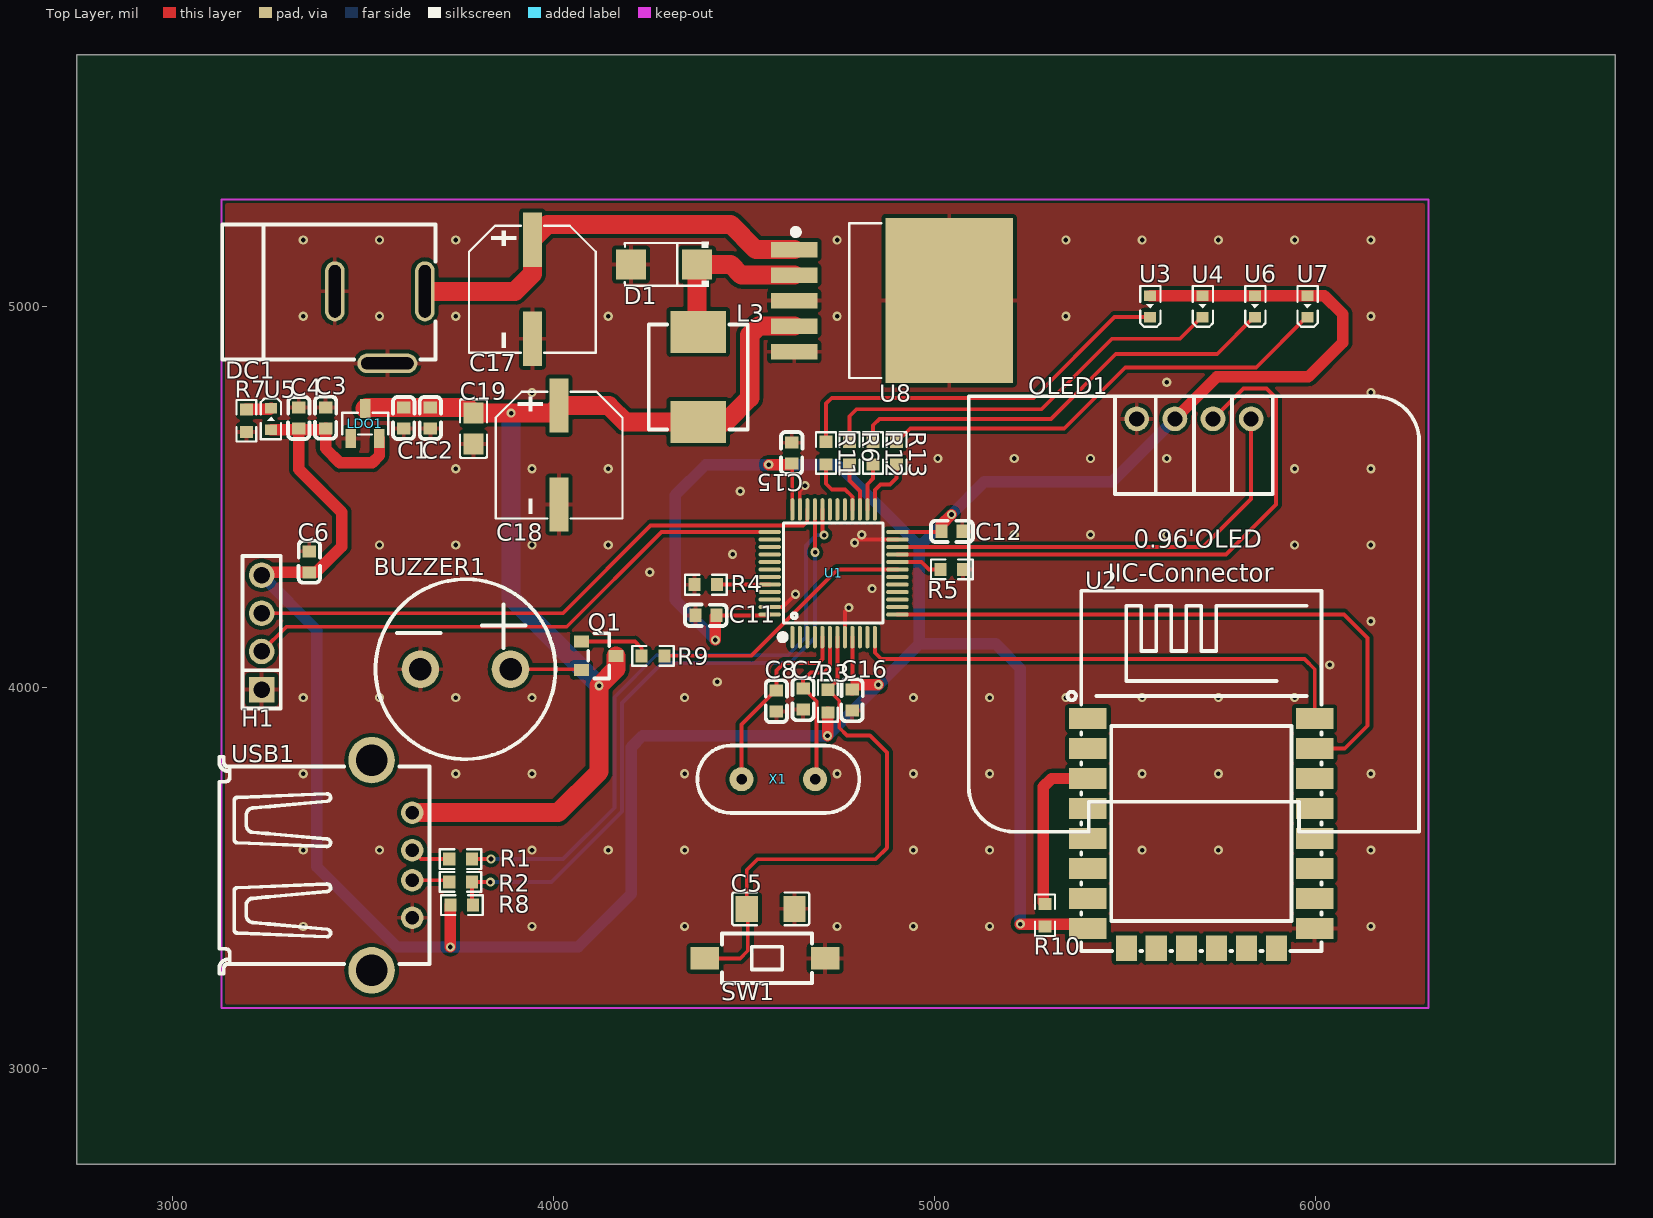
[diagram p0: Top Layer view]
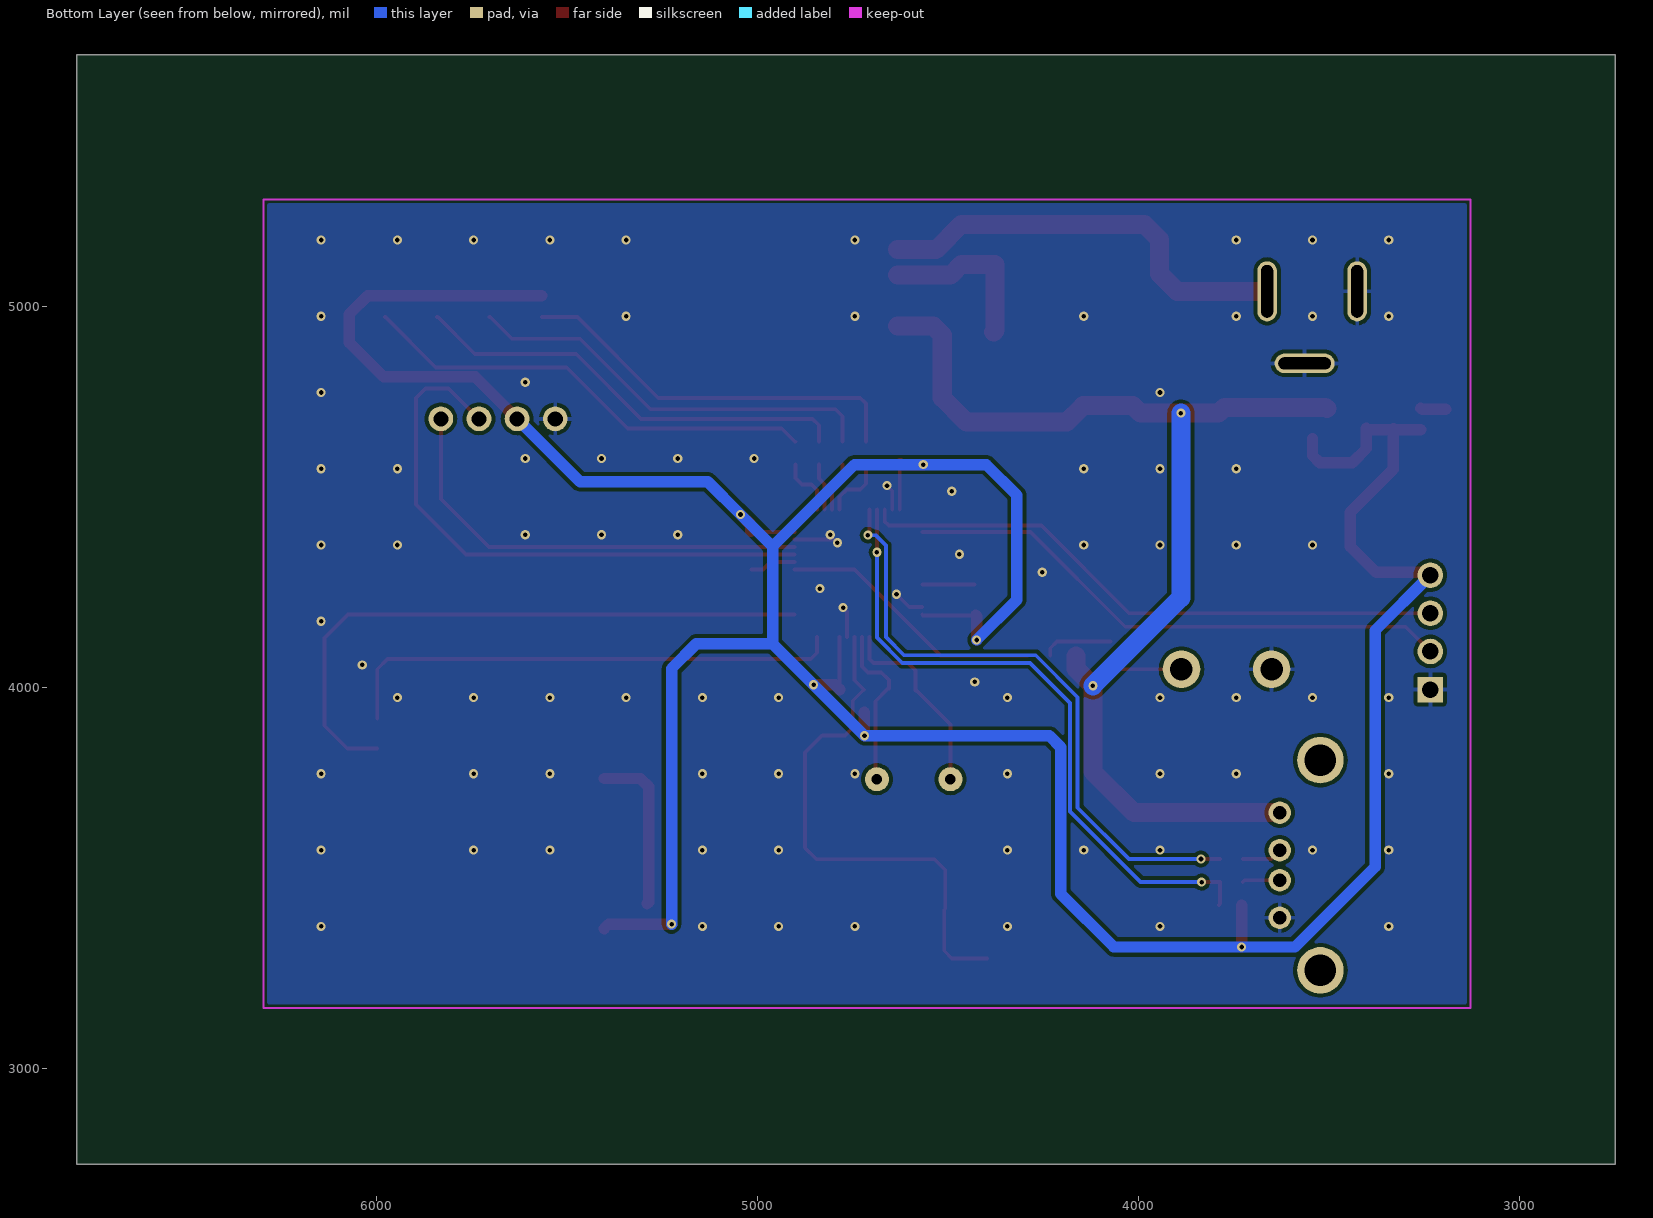
[diagram p1: Bottom Layer view, seen from below]
# Altium PCB MISC61952.pcbdoc
Units mil, origin at the board's own origin, x right, y up, seen from the top; angles counter-clockwise.
Board outline 4035 x 2910 mil, 2 copper layers (Top Layer, Bottom Layer), stack 62.206 mil thick; 47 components, 55 nets, 175 pads, 100 vias.

## Layer stack, top to bottom
Top Solder Mask Layer: solder mask 0.394, Dk 3.3
Top Layer: signal copper 1.379
Dielectric1: surface 59.449, FR4, Dk 4.5
Bottom Layer: signal copper 1.378
Bottom Solder Mask Layer: solder mask 0.394, Dk 3.3

## Board outline
6785,2750 2750,2750 2750,5660 6785,5660

## Design rules (kind name [scope] priority, off if disabled: settings)
BoardOutlineClearance copperThickness2oz_1 [All] p2 off: genericclearance=7.99 ignorepadtopadclearanceinfootprint=FALSE except(0: Arc-SplitContinuation Track-SplitContinuation SMDPad-SplitContinuation THPad-SplitContinuation Via-SplitContinuation Fill-SplitContinuation Region-SplitContinuation Poly-SplitContinuation Text-SplitContinuation Hole-SplitContinuation; 5.98: SMDPad-CutoutEdge THPad-CutoutEdge Via-CutoutEdge Fill-CutoutEdge Region-CutoutEdge Text-CutoutEdge Hole-CutoutEdge; 10: Poly-OutlineEdge Poly-CutoutEdge; 11.81: Arc-OutlineEdge Track-OutlineEdge SMDPad-OutlineEdge THPad-OutlineEdge Via-OutlineEdge Fill-OutlineEdge Region-OutlineEdge Text-OutlineEdge Hole-OutlineEdge Arc-CutoutEdge Track-CutoutEdge)
BoardOutlineClearance Plane_innerPlane_1 [All] p4 off: genericclearance=4.02 ignorepadtopadclearanceinfootprint=FALSE except(0: Arc-SplitContinuation Track-SplitContinuation SMDPad-SplitContinuation THPad-SplitContinuation Via-SplitContinuation Fill-SplitContinuation Region-SplitContinuation Poly-SplitContinuation Text-SplitContinuation Hole-SplitContinuation; 5.98: SMDPad-CutoutEdge THPad-CutoutEdge Via-CutoutEdge Fill-CutoutEdge Region-CutoutEdge Text-CutoutEdge Hole-CutoutEdge; 10: Poly-OutlineEdge Poly-CutoutEdge; 11.81: Arc-OutlineEdge Track-OutlineEdge SMDPad-OutlineEdge THPad-OutlineEdge Via-OutlineEdge Fill-OutlineEdge Region-OutlineEdge Text-OutlineEdge Hole-OutlineEdge Arc-CutoutEdge Track-CutoutEdge)
BoardOutlineClearance Copper_copperRegion_1 [All] p6 off: genericclearance=4.02 ignorepadtopadclearanceinfootprint=FALSE except(0: Arc-SplitContinuation Track-SplitContinuation SMDPad-SplitContinuation THPad-SplitContinuation Via-SplitContinuation Fill-SplitContinuation Region-SplitContinuation Poly-SplitContinuation Text-SplitContinuation Hole-SplitContinuation; 5.98: SMDPad-CutoutEdge THPad-CutoutEdge Via-CutoutEdge Fill-CutoutEdge Region-CutoutEdge Text-CutoutEdge Hole-CutoutEdge; 10: Poly-OutlineEdge Poly-CutoutEdge; 11.81: Arc-OutlineEdge Track-OutlineEdge SMDPad-OutlineEdge THPad-OutlineEdge Via-OutlineEdge Fill-OutlineEdge Region-OutlineEdge Text-OutlineEdge Hole-OutlineEdge Arc-CutoutEdge Track-CutoutEdge)
BoardOutlineClearance copperThickness1oz_1 [All] p8: genericclearance=4.02 ignorepadtopadclearanceinfootprint=FALSE except(0: Arc-SplitContinuation Track-SplitContinuation SMDPad-SplitContinuation THPad-SplitContinuation Via-SplitContinuation Fill-SplitContinuation Region-SplitContinuation Poly-SplitContinuation Text-SplitContinuation Hole-SplitContinuation; 5.98: SMDPad-CutoutEdge THPad-CutoutEdge Via-CutoutEdge Fill-CutoutEdge Region-CutoutEdge Text-CutoutEdge Hole-CutoutEdge; 10: Poly-OutlineEdge Poly-CutoutEdge; 11.81: Arc-OutlineEdge Track-OutlineEdge SMDPad-OutlineEdge THPad-OutlineEdge Via-OutlineEdge Fill-OutlineEdge Region-OutlineEdge Text-OutlineEdge Hole-OutlineEdge Arc-CutoutEdge Track-CutoutEdge)
Clearance copperThickness2oz [All] p1 off: gap=7.99 ignorepadtopadclearanceinfootprint=FALSE except(5.98: SMDPad-Track SMDPad-SMDPad THPad-Track SMDPad-THPad THPad-THPad Track-Via SMDPad-Via THPad-Via Via-Via Fill-Track Region-Track Fill-SMDPad Region-SMDPad Fill-THPad Region-THPad Fill-Via Region-Via Fill-Fill Fill-Region Region-Region Arc-Track Arc-SMDPad Arc-THPad Arc-Via Fill-Arc Region-Arc Arc-Arc Text-Track SMDPad-Text Text-THPad Text-Via Fill-Text Region-Text Arc-Text Text-Text Hole-Track Hole-SMDPad Hole-THPad Hole-Via Fill-Hole Region-Hole Hole-Arc Hole-Text; 10: Poly-Track Poly-SMDPad Poly-THPad Poly-Via Poly-Fill Poly-Region Poly-Poly Poly-Arc Poly-Text Poly-Hole)
Clearance Plane_innerPlane [All] p3 off: gap=4.02 ignorepadtopadclearanceinfootprint=FALSE except(5.98: SMDPad-Track SMDPad-SMDPad THPad-Track SMDPad-THPad THPad-THPad Track-Via SMDPad-Via THPad-Via Via-Via Fill-Track Region-Track Fill-SMDPad Region-SMDPad Fill-THPad Region-THPad Fill-Via Region-Via Fill-Fill Fill-Region Region-Region Arc-Track Arc-SMDPad Arc-THPad Arc-Via Fill-Arc Region-Arc Arc-Arc Text-Track SMDPad-Text Text-THPad Text-Via Fill-Text Region-Text Arc-Text Text-Text Hole-Track Hole-SMDPad Hole-THPad Hole-Via Fill-Hole Region-Hole Hole-Arc Hole-Text; 10: Poly-Track Poly-SMDPad Poly-THPad Poly-Via Poly-Fill Poly-Region Poly-Poly Poly-Arc Poly-Text Poly-Hole)
Clearance Copper_copperRegion [All] p5 off: gap=4.02 ignorepadtopadclearanceinfootprint=FALSE except(5.98: SMDPad-Track SMDPad-SMDPad THPad-Track SMDPad-THPad THPad-THPad Track-Via SMDPad-Via THPad-Via Via-Via Fill-Track Region-Track Fill-SMDPad Region-SMDPad Fill-THPad Region-THPad Fill-Via Region-Via Fill-Fill Fill-Region Region-Region Arc-Track Arc-SMDPad Arc-THPad Arc-Via Fill-Arc Region-Arc Arc-Arc Text-Track SMDPad-Text Text-THPad Text-Via Fill-Text Region-Text Arc-Text Text-Text Hole-Track Hole-SMDPad Hole-THPad Hole-Via Fill-Hole Region-Hole Hole-Arc Hole-Text; 10: Poly-Track Poly-SMDPad Poly-THPad Poly-Via Poly-Fill Poly-Region Poly-Poly Poly-Arc Poly-Text Poly-Hole)
Clearance copperThickness1oz [All] p7: gap=4.02 ignorepadtopadclearanceinfootprint=FALSE except(5.98: SMDPad-Track SMDPad-SMDPad THPad-Track SMDPad-THPad THPad-THPad Track-Via SMDPad-Via THPad-Via Via-Via Fill-Track Region-Track Fill-SMDPad Region-SMDPad Fill-THPad Region-THPad Fill-Via Region-Via Fill-Fill Fill-Region Region-Region Arc-Track Arc-SMDPad Arc-THPad Arc-Via Fill-Arc Region-Arc Arc-Arc Text-Track SMDPad-Text Text-THPad Text-Via Fill-Text Region-Text Arc-Text Text-Text Hole-Track Hole-SMDPad Hole-THPad Hole-Via Fill-Hole Region-Hole Hole-Arc Hole-Text; 10: Poly-Track Poly-SMDPad Poly-THPad Poly-Via Poly-Fill Poly-Region Poly-Poly Poly-Arc Poly-Text Poly-Hole)
DiffPairsRouting differentialPair [All] p1: maxlimit=6 minlimit=6 mostfreqgap=6 toplayer_minwidth=5 toplayer_prefwidth=10 toplayer_maxwidth=100 toplayer_mingap=6 toplayer_prefgap=6 toplayer_maxgap=6 bottomlayer_minwidth=5 bottomlayer_prefwidth=10 bottomlayer_maxwidth=100 bottomlayer_mingap=6 bottomlayer_prefgap=6 bottomlayer_maxgap=6 maxuncoupledlength=10
HoleToHoleClearance otherClearance [All] p1: gap=11.8 allowstackedmicrovias=TRUE
Length netLength [All] p1: minlimit=0 maxlimit=0
PasteMaskExpansion pasteMaskExpansion [All] p1: expansion=0
PlaneConnect innerPlane [All] p1: planeconnectstyle=Relief reliefexpansion=20 reliefentries=4 reliefconductorwidth=10 reliefairgap=10
PolygonConnect copperRegion [All] p1: connectstyle=Relief reliefconductorwidth=10 reliefentries=4 polygonreliefangle="90 Angle" airgapwidth=10 via.connectstyle=Relief via.reliefconductorwidth=10 via.reliefentries=4 via.polygonreliefangle="90 Angle" via.airgapwidth=10
RoutingVias viaSize [All] p1: holewidth=12.01 width=24.02 viastyle="Through Hole" minholewidth=11.81 minwidth=19.68 maxholewidth=248.03 maxwidth=393.7
SolderMaskExpansion solderMaskExpansion [IsVia] p1: expansion=-1000 istentingtop=TRUE
SolderMaskExpansion solderMaskExpansion [All] p2: expansion=2 istentingtop=FALSE
Width copperThickness2oz_2 [All] p1 off: maxlimit=100 minlimit=8 preferedwidth=10
Width copperThickness1oz_2 [All] p2: maxlimit=100 minlimit=5 preferedwidth=10

## Components (designator, comment, footprint, x,y, rotation, side; value= is the part's Value field where it differs from the comment)
BUZZER1 "buzzer" BUZ-TH_BD12.0-P6.00-D0.9-RD 3769.57,4048.51 r0 top
C1 "10uF" C0603 3607.6,4707.62 r90 top
C2 "100nF" C0603 3677.6,4707.62 r90 top
C3 "100nF" C0603 3402.6,4707.62 r270 top
C4 "10uF" C0603 3332.38,4707.01 r270 top
C5 "100uF" C1206 4570,3420 r180 top
C6 "100nF" C0603 3360,4330 r270 top
C7 "20pF" C0603 4655,3970 r90 top
C8 "20pF" C0603 4585,3965 r90 top
C11 "100nF" C0603 4400.2,4189.59 r0 top
C12 "100nF" C0603 5045,4410 r180 top
C15 "100nF" C0603 4625,4615 r270 top
C16 "4.7nF" C0603 4783.39,3967.44 r90 top
C17 "" CAP-SMD_BD8.0-L8.3-W8.3-RD 3945,5045 r90 top
C18 "" CAP-SMD_BD8.0-L8.3-W8.3-RD 4015,4610 r90 top
C19 "" C0805 3790.55,4679.45 r270 top
D1 "" SMA_L4.3-W2.6-LS5.2-RD 4290,5110 r180 top
DC1 "" DC-2.0 3540,5050 r180 top
H1 "" HDR-TH_4P-P2.54-V-M 3235,4145 r90 top
L3 "" IND-SMD_L7.0-W6.6 4380,4815 r270 top
LDO1 "SC662K-3.3V" SOT-23-3_L2.9-W1.3-P1.90-LS2.4-BR 3506.61,4692.62 r270 top
OLED1 "" 0.96OLED_4P 5680,4705 r0 top
Q1 "" S8050_SOT-23 4119.17,4083.51 r180 top
R1 "20Ω" R0603 3756.64,3550.63 r0 top
R2 "20Ω" R0603 3756.64,3490.63 r0 top
R3 "1kΩ" R0603 4720,3965 r270 top
R4 "10kΩ" R0603 4400,4270 r0 top
R5 "10kΩ" R0603 5045,4310 r180 top
R6 "510Ω" R0603 4776.67,4615.37 r270 top
R7 "510Ω" R0603 3195,4700 r270 top
R8 "1.5kΩ" R0603 3760,3430 r0 top
R9 "10K" R0603 4261.34,4083.51 r180 top
R10 "10K" R0603 5289.34,3403.15 r90 top
R11 "510Ω" R0603 4715,4615.37 r270 top
R12 "510Ω" R0603 4838.33,4615.37 r270 top
R13 "510Ω" R0603 4900,4615.37 r270 top
SW1 "TS-1101-C-W" SW-SMD_L6.0-W3.3-LS8.0 4555,3290 r180 top
U1 "STM32F103C8T6" LQFP-48_L7.0-W7.0-P0.50-LS9.0-BL 4735,4300 r0 top
U2 "ESP8266" WIFIM-SMD_ESP-12F-ESP8266MOD 5699.34,3618.15 r270 top
U3 "42-51/GHC-YW2X2K/3T" LED-SMD_L1.6-W0.8-FD_GREEN-1 5565,5000 r270 top
U4 "42-51/GHC-YW2X2K/3T" LED-SMD_L1.6-W0.8-FD_GREEN-1 5702.45,5000 r270 top
U5 "42-51/GHC-YW2X2K/3T" LED-SMD_L1.6-W0.8-FD_GREEN-1 3260,4705 r90 top
U6 "42-51/GHC-YW2X2K/3T" LED-SMD_L1.6-W0.8-FD_GREEN-1 5839.89,5000 r270 top
U7 "42-51/GHC-YW2X2K/3T" LED-SMD_L1.6-W0.8-FD_GREEN-1 5977.34,5000 r270 top
U8 "LM2596S-5.0" TO-263-5_L10.2-W8.9-P1.70-BR 4835,5015 r180 top
USB1 "" "USB_ Type-A" 3415,3535 r270 top
X1 "8MHz" OSC-TH_L10.0-W4.5-P5.00 4590,3760 r90 top

## Footprints (in the part's own frame and the unit in brackets; to place one, negate y for a bottom-side part, rotate by r counter-clockwise, add the part's x,y. Pads: shape width x height; smd on the part's side, far side on the other; paste and mask are expansions set on the pad)
0.96OLED_4P [mm]
  round 1.65 hole 1 copper offset 0,0: 1(-3.81,-0.001) 2(-1.27,0.002) 3(1.27,0.002) 4(3.81,0.002)
  silkscreen extent -15,-27.5 15,1.5
BUZ-TH_BD12.0-P6.00-D0.9-RD [mm]
  round 2.5 hole 1.5 paste+0 mask+0.05: 1(-3,0) 2(3,0)
  silkscreen extent -5.99,-5.99 5.99,5.99
C0603 [mm]
  rect 0.8x0.9 smd: 1(-0.7,0) 2(0.7,0)
  silkscreen extent -1.41,-0.71 1.39,0.72
C0805 [mm]
  rect 1.41x1.35 smd paste-100 mask+0.051: 1(-1.03,0) 2(1.03,0)
  silkscreen extent -1.96,-0.9 1.96,0.9
C1206 [mm]
  rect 1.485x1.728 smd paste-100 mask+0.051: 1(-1.593,0) 2(1.593,0)
  silkscreen extent -2.56,-1.09 2.56,1.09
CAP-SMD_BD8.0-L8.3-W8.3-RD [mm]
  rect 3.61x1.26 smd paste+0 mask+0.051: 1(3.295,0) 2(-3.295,0)
  silkscreen extent -4.23,-4.23 4.23,4.23
DC-2.0 [mil]
  oval 157.5x51.2 hole 31.5 slot 137.8 at 0 deg paste+0 mask+2: 2(-24.7,199.5)
  oval 51.2x157.5 hole 31.5 slot 137.8 at 90 deg paste+0 mask+2: 3(113.1,10.5) 4(-123.1,10.5)
  silkscreen extent -151,-165 408,190
HDR-TH_4P-P2.54-V-M [mm]
  rect 1.7x1.7 hole 1.1: 1(-3.81,0)
  round 1.7 hole 1.1: 2(-1.27,0) 3(1.27,0) 4(3.81,0)
  silkscreen extent -5.08,-1.27 5.08,1.27
IND-SMD_L7.0-W6.6 [mil]
  rect 110.2x145.7 smd paste+0 mask+2: 1(-118.1,0) 2(118.1,0)
  silkscreen extent -138,-130 138,130
LED-SMD_L1.6-W0.8-FD_GREEN-1 [mm]
  rect 0.7x0.8 smd: 1(-0.715,0) 2(0.715,0)
  silkscreen extent -1.35,-0.65 1.35,0.7
LQFP-48_L7.0-W7.0-P0.50-LS9.0-BL [mm]
  oval 0.27x1.5 smd paste+0 mask+0.05: 1(-2.75,-4.25) 2(-2.25,-4.25) 3(-1.75,-4.25) 4(-1.25,-4.25) 5(-0.75,-4.25) 6(-0.25,-4.25) 7(0.25,-4.25) 8(0.75,-4.25) 9(1.25,-4.25) 10(1.75,-4.25) 11(2.25,-4.25) 12(2.75,-4.25) 25(2.75,4.25) 26(2.25,4.25) 27(1.75,4.25) 28(1.25,4.25) 29(0.75,4.25) 30(0.25,4.25) 31(-0.25,4.25) 32(-0.75,4.25) 33(-1.25,4.25) 34(-1.75,4.25) 35(-2.25,4.25) 36(-2.75,4.25)
  oval 1.5x0.27 smd paste+0 mask+0.05: 13(4.25,-2.75) 14(4.25,-2.25) 15(4.25,-1.75) 16(4.25,-1.25) 17(4.25,-0.75) 18(4.25,-0.25) 19(4.25,0.25) 20(4.25,0.75) 21(4.25,1.25) 22(4.25,1.75) 23(4.25,2.25) 24(4.25,2.75) 37(-4.25,2.75) 38(-4.25,2.25) 39(-4.25,1.75) 40(-4.25,1.25) 41(-4.25,0.75) 42(-4.25,0.25) 43(-4.25,-0.25) 44(-4.25,-0.75) 45(-4.25,-1.25) 46(-4.25,-1.75) 47(-4.25,-2.25) 48(-4.25,-2.75)
  silkscreen extent -3.59,-4.46 3.3,3.34
OSC-TH_L10.0-W4.5-P5.00 [mm]
  round 1.6 hole 0.7: 1(0,2.45) 2(0,-2.45)
  silkscreen extent -2.25,-5.39 2.25,5.39
R0603 [mil]
  rect 31.75x34.02 smd paste-3937.01 mask+2: 1(-29.66,0) 2(29.66,0)
  silkscreen extent -55,-26 55,26
S8050_SOT-23 [mm]
  rect 1x0.8 smd paste+0 mask+0.051: 1(1.15,-0.95) 2(1.15,0.95) 3(-1.15,0)
  silkscreen extent -0.7,-1.5 0.7,1.5
SMA_L4.3-W2.6-LS5.2-RD [mm]
  rect 2x2 smd paste+0 mask+0.051: 1(-2.2,0) 2(2.2,0)
  silkscreen extent -2.98,-1.5 2.6,1.5
SOT-23-3_L2.9-W1.3-P1.90-LS2.4-BR [mm]
  rect 1.25x0.7 smd: 1(1,-0.95) 2(1,0.95) 3(-1,0)
  silkscreen extent -0.73,-1.53 0.73,1.53
SW-SMD_L6.0-W3.3-LS8.0 [mm]
  rect 1.9x1.5 smd: 1(-4,0) 2(4,0)
  silkscreen extent -3.14,-1.67 2.86,1.63
TO-263-5_L10.2-W8.9-P1.70-BR [mm]
  rect 3.083x1.02 smd: 1(5.16,-3.4) 2(5.16,-1.7) 3(5.16,0) 4(5.16,1.7) 5(5.16,3.4)
  rect 8.5x11 smd: 6(-5.16,0)
  silkscreen extent -0.66,-5.16 5.26,5.16
"USB_ Type-A" [mm]
  round 1.5 hole 0.9 copper offset 0,0 paste+0 mask+0.051: 1(-3.484,5.461) 4(3.516,5.461)
  round 1.5 hole 0.9 paste+0 mask+0.051: 2(-0.984,5.461) 3(1.016,5.461)
  round 3.1 hole 2.1 paste+0 mask+0.051: SH1(7.016,2.751) SH2(-6.984,2.751)
  silkscreen extent -7.2,-7.4 7.24,6.6
WIFIM-SMD_ESP-12F-ESP8266MOD [mm]
  rect 1.4x2.5 smd: 1(-7.651,-7.551) 2(-5.651,-7.551) 3(-3.651,-7.551) 4(-1.651,-7.551) 5(0.349,-7.551) 6(2.349,-7.551) 7(4.349,-7.551) 8(6.349,-7.551) 9(6.349,7.549) 10(4.349,7.55) 11(2.349,7.551) 12(0.349,7.551) 13(-1.651,7.55) 14(-3.651,7.551) 15(-5.651,7.55) 16(-7.651,7.551)
  rect 1.7x1.4 smd: 17(7.651,-5) 18(7.649,-3.002) 19(7.65,-1.003) 20(7.65,0.997) 21(7.65,2.997) 22(7.65,4.997)
  silkscreen extent -16.15,-8.92 7.85,8

## Via types
v1: diameter 24.02, hole 12, Top Layer to Bottom Layer, 100 vias

## Nets (pads, with @x,y where several pads share a name; then routed paths per layer and width w, separated by ;. In a path a pad name is that pad's centre, name@x,y a point inside that pad or via, vN(x,y) a via of type N, cw(c..) or ccw(c..) an arc to the next point about the centre after c; other vN are vias at no path point)
3V3: C3.2 C4.2 C6.2 C11.2 C12.2 C15.2 C16.2 H1.4 LDO1.2 OLED1.2 R3.2 R8.1 R10.1 U1.9 U1.24 U1.36 U1.48 U2.8 U3.1 U4.1 U5.1 U6.1 U7.1 | length 9508.2
  Top Layer w10: C11.2 4565.54,4189.59 U1.48 ; C15.2 4626.73,4585.71 U1.36 ; C16.2@4784.21,3995.82 U1.9 ; U1.24 5015.71,4408.27 C12.2
  Top Layer w30: H1.4 3242.44,4302.44 C6.2 3377.44,4302.44 3445,4370 3445,4460 3332.38,4572.62 C4.2@3332.38,4676.85 ; U5.1 C4.2@3332.38,4676.85 ; C4.2 C4.2@3332.38,4676.85 ; LDO1.2 3544.01,4609.01 3525,4590 3440,4590 3402.6,4627.4 C3.2 3399.39,4676.85 C4.2@3332.38,4676.85 ; v1(3730,3320) 3730,3429.66 R8.1 ; v1(4425,4125) 4425,4186.83 C11.2 ; v1(4565,4585) 4622.56,4585 C15.2 ; v1(4719.02,3874.02) 4720,3875 R3.2 ; C16.2 4784.21,3995.82 4795.89,4007.5 v1(4852.5,4007.5) ; C12.2 5017.44,4427.44 v1(5044.15,4454.15) ; v1(5225,3380) 5390.25,3380 U2.8 ; U3.1 U4.1 U6.1 U7.1 6021.85,5028.15 6070,4980 6070,4905 5980,4815 5739.95,4815 OLED1.2@5630,4705.05
  Bottom Layer w30: H1.4 3380,4150 3380,3530 3590,3320 v1(3730,3320) 4065,3320 4204.02,3459.02 4204.02,3844.02 4234.02,3874.02 v1(4719.02,3874.02) v1(4852.5,4007.5) 4960,4115 ; v1(4425,4125) 4320,4230 4320,4505 4400,4585 v1(4565,4585) 4745,4585 4960,4370 ; v1(5225,3380) 5225,4050 5160,4115 4960,4115 ; OLED1.2@5630,4705.05 5464.95,4540 5130,4540 v1(5044.15,4454.15) 4960,4370 ; 4960,4115 4960,4370
$1N2679: R1.1 USB1.2 | length 106.5
  Top Layer w10: USB1.2 3653.11,3550.63 R1.1
$1N2682: R2.1 USB1.3 | length 98.8
  Top Layer w10: USB1.3 3722.61,3495 R2.1
$1N5665: R7.1 U5.2 | length 66.4
  Top Layer w30: R7.1 3256.51,4729.66 U5.2
$1N13486: Q1.1 R9.2 | length 184.9
  Top Layer w10: Q1.1 4214.08,4120.92 4231.68,4103.32 R9.2
$1N13487: BUZZER1.2 Q1.2 | length 187.2
  Top Layer w10: BUZZER1.2 4071.49,4048.51 Q1.2
$1N13495: R10.2 U2.3 | length 435.1
  Top Layer w30: R10.2 5285,3437.16 5285,3740 5306.88,3761.88 U2.3
$1N13498: R11.1 U3.2 | length 1043.9
  Top Layer w10: R11.1 4715,4745 4730,4760 5260,4760 5471.85,4971.85 U3.2
$1N13500: R6.1 U4.2 | length 1100.2
  Top Layer w10: R6.1 4776.67,4711.67 4795,4730 5280,4730 5465,4915 5643.63,4915 5700.48,4971.85 U4.2
$1N13501: R12.1 U6.2 | length 1162.3
  Top Layer w10: R12.1 4838.33,4688.33 4855,4705 5305,4705 5475,4875 5741.08,4875 5837.93,4971.85 U6.2
$1N13503: R13.1 U7.2 | length 1212.7
  Top Layer w10: R13.1 4901.13,4645.03 4936.11,4680 5340,4680 5500,4840 5843.52,4840 5975.37,4971.85 U7.2
$1N13509: C17.1 DC1.4 U8.1 | length 1121.4
  Top Layer w50: DC1.4 3899.5,5039.5 3945,5085 C17.1 3985.28,5215 4465,5215 4531.14,5148.86 U8.1
$1N13514: D1.1 L3.1 U8.2 | length 445.2
  Top Layer w50: L3.1 4376.61,4936.49 D1.1 4465,5110 4493.07,5081.93 U8.2
+5V: C1.2 C2.2 C18.1 C19.1 L3.2 LDO1.3 Q1.3 U8.4 USB1.1 | length 3026.6
  Top Layer w50: LDO1.3 3509.8,4735.18 C1.2 C2.2 3775.37,4735.18 C19.1 v1(3889.39,4720) 3995.28,4720 C18.1 4145.28,4739.72 4188.1,4696.9 L3.2 4451.9,4696.9 4515,4760 4515,4925 4538.07,4948.07 U8.4 ; USB1.1 4012.17,3672.17 4120,3780 v1(4120,4005) 4164.44,4049.44 Q1.3
  Bottom Layer w50: v1(3889.39,4720) 3889.39,4235.61 v1(4120,4005)
BOOT0: R4.2 U1.44 | length 138.2
  Top Layer w10: R4.2 4430.13,4270.47 U1.44
BOOT1: R5.2 U1.20 | length 121.1
  Top Layer w10: U1.20 4965.47,4329.53 4985,4310 R5.2
CLK: H1.2 U1.37 | length 1462.4
  Top Layer w10: H1.2 3300,4160 4035,4160 4283.27,4408.27 U1.37
DIO: H1.3 U1.34 | length 1562.2
  Top Layer w10: H1.3 4025,4195 4255,4425 4655,4425 4666.1,4436.1 U1.34
GND: BUZZER1.1 C1.1 C2.1 C3.1 C4.1 C5.1 C6.1 C7.1 C8.1 C11.1 C12.1 C15.1 C16.1 C17.2 C18.2 C19.2 D1.2 DC1.2 DC1.3 H1.1 LDO1.1 OLED1.1 R4.1 R5.1 R7.2 SW1.1 U1.8 U1.23 U1.35 U1.47 U2.9 U8.3 U8.5 U8.6 USB1.4 | length 347.1
  Top Layer w10: U1.47 4601.42,4211.42 v1(4635,4245) ; U1.35 4646.42,4516.42 v1(4660,4530) ; U1.8 4764.53,4199.53 v1(4775,4210) ; v1(4790,4380) 4798.58,4388.58 U1.23
  other v1: 3344.1,3374.1 3944.1,3374.1 4344.1,3374.1 4744.1,3374.1 4944.1,3374.1 5144.1,3374.1 6144.1,3374.1 3344.1,3574.1 3544.1,3574.1 3944.1,3574.1 4144.1,3574.1 4344.1,3574.1 4944.1,3574.1 5144.1,3574.1 5544.1,3574.1 5744.1,3574.1 6144.1,3574.1 3344.1,3774.1 3744.1,3774.1 3944.1,3774.1 4344.1,3774.1 4744.1,3774.1 4944.1,3774.1 5144.1,3774.1 5544.1,3774.1 5744.1,3774.1 6144.1,3774.1 3344.1,3974.1 3544.1,3974.1 3744.1,3974.1 3944.1,3974.1 4344.1,3974.1 4944.1,3974.1 5144.1,3974.1 5344.1,3974.1 5544.1,3974.1 5744.1,3974.1 5944.1,3974.1 4430,4015 6035.98,4059.72 6144.1,4174.1 4835.98,4259.72 4252.69,4302.61 4470,4350 3544.1,4374.1 3744.1,4374.1 3944.1,4374.1 4144.1,4374.1 5944.1,4374.1 6144.1,4374.1 4808.63,4400.98 5208.63,4400.98 5408.63,4400.98 5608.63,4400.98 4490,4515 3744.1,4574.1 3944.1,4574.1 4144.1,4574.1 5944.1,4574.1 6144.1,4574.1 5008.63,4600.98 5208.63,4600.98 5408.63,4600.98 5608.63,4600.98 3944.1,4774.1 6144.1,4774.1 5608.63,4800.98 3344.1,4974.1 3544.1,4974.1 3744.1,4974.1 4144.1,4974.1 4744.1,4974.1 5344.1,4974.1 6144.1,4974.1 3344.1,5174.1 3544.1,5174.1 3744.1,5174.1 4744.1,5174.1 5344.1,5174.1 5544.1,5174.1 5744.1,5174.1 5944.1,5174.1 6144.1,5174.1
OSC32-IN: U1.3
OSC32-OUT: U1.4
OSC-IN: C8.2 U1.5 X1.1 | length 514.3
  Top Layer w10: X1.1 4493.54,3903.07 4583.03,3992.56 C8.2 4585,4045 4605,4065 4695,4065 4705.47,4075.47 U1.5
OSC-OUT: C7.2 U1.6 X1.2 | length 447.6
  Top Layer w10: X1.2@4666.46,3760 4690,3783.54 4690,3964.53 4656.97,3997.56 C7.2 4655,4020 4675,4040 4710,4040 4725.16,4055.16 U1.6
PA0: U1.10
PA1: U1.11
PA2: U1.12 U2.16 | length 1341.3
  Top Layer w10: U1.12 4843.27,4091.73 4860,4075 5970,4075 5996.61,4048.39 U2.16
PA3: U1.13 U2.15 | length 1651.2
  Top Layer w10: U1.13 6073.27,4191.73 6135,4130 6135,3900 6075.62,3840.62 U2.15
PA4: U1.14
PA5: U1.15
PA6: U1.16
PA7: U1.17
PA8: U1.29
PA9: U1.30
PA10: U1.31
PA11: R1.2 U1.32 | length 1655.1
  Top Layer w10: R1.2 v1(3836.43,3550.63) ; U1.32 4705.47,4404.53 v1(4710,4400)
  Bottom Layer w10: v1(3836.43,3550.63) 4025.63,3550.63 4160,3685 4160,3975 4270,4085 4615,4085 4662.8,4132.8 4662.8,4372.62 4690.18,4400 v1(4710,4400)
PA12: R2.2 R8.2 U1.33 | length 1731.3
  Top Layer w10: R8.2 3786.3,3433.36 R2.2 3786.93,3490 v1(3835,3490) ; U1.33 4686.58,4466.53 v1(4686.58,4355)
  Bottom Layer w10: v1(3835,3490) 3995,3490 4180,3675 4180,3960 4285,4065 4620,4065 4686.58,4131.58 v1(4686.58,4355)
PA15: U1.38
PB0: U1.18
PB1: R9.1 U1.19 | length 705.1
  Top Layer w10: R9.1 4518.51,4083.51 4744.84,4309.84 U1.19
PB3: U1.39
PB4: U1.40
PB5: U1.41
PB6: U1.42
PB7: U1.43
PB8: U1.45
PB9: U1.46
PB10: OLED1.3 U1.21 | length 1535.3
  Top Layer w10: U1.21 5764.21,4349.21 5895,4480 5895,4760 5870,4785 5809.95,4785 OLED1.3@5730,4705.05
PB11: OLED1.4 U1.22 | length 1190
  Top Layer w10: U1.22 5703.9,4368.9 5830,4495 OLED1.4@5830,4705.05
PB12: R13.2 U1.25 | length 156.5
  Top Layer w10: U1.25 4843.27,4518.27 4858.12,4533.12 4883.12,4533.12 4900,4550 R13.2
PB13: R12.2 U1.26 | length 124.5
  Top Layer w10: U1.26 4823.58,4533.58 4838.33,4548.33 R12.2
PB14: R6.2 U1.27 | length 129.7
  Top Layer w10: R6.2 4776.67,4543.33 4803.9,4516.1 U1.27
PB15: R11.2 U1.28 | length 167.6
  Top Layer w10: R11.2 4715,4535 4730,4520 4765,4520 4784.21,4500.79 U1.28
PC13: U1.2
REST: C5.2 R3.1 SW1.2 U1.7 | length 1388.8
  Top Layer w10: SW1.2 4490,3290 4510,3310 4510,3417.3 C5.2 4507.3,3522.3 4535,3550 4845,3550 4875,3580 4875,3830 4830,3875 4770,3875 4750,3895 4750,3965.79 4721.13,3994.66 R3.1 4744.84,4019.5 U1.7
VBAT: U1.1
pads on no net: U2.1 U2.2 U2.4 U2.5 U2.6 U2.7 U2.10 U2.11 U2.12 U2.13 U2.14 U2.17 U2.18 U2.19 U2.20 U2.21 U2.22 USB1.SH1 USB1.SH2

## Polygon pours and split planes (outlines as drawn)
GND on Top Layer (solid, remove dead copper, pour order 0): 3000,5410 3000,3010 6480,3010 6480,5410
GND on Bottom Layer (solid, remove dead copper, pour order 2): 3065,5400 3065,3000 6535,3000 6535,5400

## Keep-outs
Board Outline Layer:
  lines w5: 3130,3160 3130,5280 6295,5280 6295,3160 3130,3160